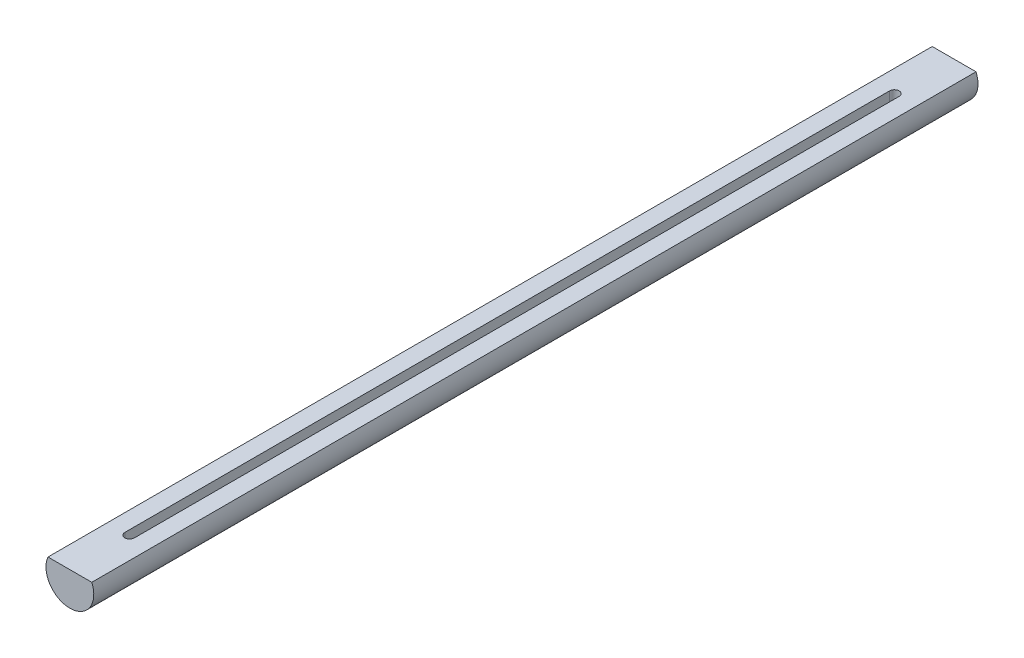
SolidWorks part; units mm, degrees
ref_plane "前视基准面" through (0, 0, 0) normal (0, 0, 1) x (1, 0, 0)
ref_plane "上视基准面" through (0, 0, 0) normal (0, 1, 0) x (1, 0, 0)
ref_plane "右视基准面" through (0, 0, 0) normal (1, 0, 0) x (0, 0, -1)
sketch "草图3" plane through (0, 0, 0) normal (0, 0, 1) x (1, 0, 0)
  circle A0 centre (0, 0) radius 10
  dimension "D1" = 20
extrude "凸台-拉伸3" add sketch "草图3" along normal mid plane 370
sketch "草图4" plane through (0, 0, 0) normal (0, 1, 0) x (1, 0, 0)
  line L0 (0, -160) -> (0, 160) construction
  line L1 (-2, -160) -> (-2, 160)
  line L2 (2, -160) -> (2, 160)
  line L3 (10, 185) -> (-10, 185) construction
  arc A0 (-2, -160) -> (2, -160) centre (0, -160) ccw
  arc A1 (2, 160) -> (-2, 160) centre (0, 160) ccw
  point P2 (0, 0)
  dimension "D1" = 2
  dimension "D2" = 25
extrude "切除-拉伸1" cut sketch "草图4" against normal mid plane 25
sketch "草图5" plane through (0, 0, 0) normal (1, 0, 0) x (0, 0, -1)
  line L1 (-185, 4) -> (185, 4)
  line L2 (-185, 4) -> (-185, 24)
  line L3 (-185, 24) -> (185, 24)
  line L4 (185, 4) -> (185, 24)
  line L6 (185, -10) -> (185, 10) construction
  line L7 (-185, 10) -> (-185, -10) construction
  dimension "D1" = 4
  dimension "D3" = 20
extrude "切除-拉伸2" cut sketch "草图5" against normal mid plane 20
